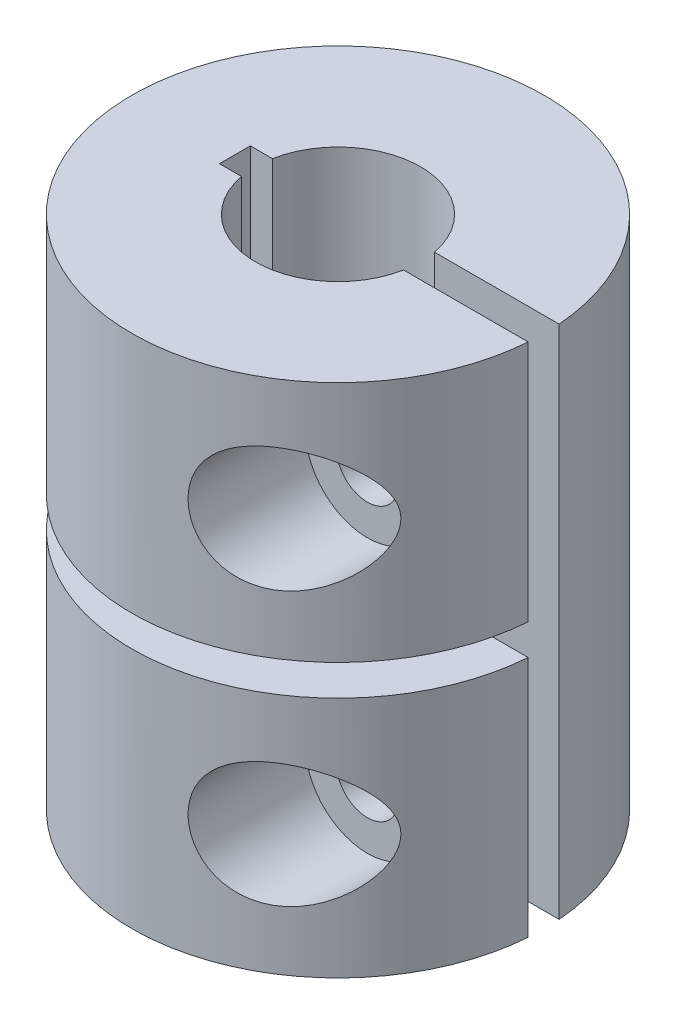
from build123d import *

# Parameters (mm, degrees)
SKETCH2_R               = 10
SKETCH2_R_2             = 4
BOSS_EXTRUDE1_DEPTH     = 25
CUT_EXTRUDE1_DEPTH      = 25
CUT_EXTRUDE1_DEPTH_BACK = 25
SKETCH3_W               = 10.75
SKETCH3_H               = 1.5
SKETCH4_W               = 17.874578158
SKETCH4_H               = 1.5
CUT_EXTRUDE2_DEPTH      = 29.722813233
SKETCH5_R               = 3
CUT_EXTRUDE3_DEPTH      = 6
SKETCH6_R               = 1.5
CUT_EXTRUDE4_DEPTH      = 4
M3_TAPPED_HOLE3_D       = 2.5


with BuildPart() as part:
    # Sketch2 → Boss-Extrude1 (new body)
    with BuildSketch(Plane(origin=(0, 0, 0), x_dir=(1, 0, 0), z_dir=(0, 1, 0))):
        with Locations(Location((0, 0, 0), (0, 0, 270))):
            Circle(SKETCH2_R)
        with Locations(Location((0, 0, 0), (0, 0, 270))):
            Circle(SKETCH2_R_2, mode=Mode.SUBTRACT)
    extrude(amount=BOSS_EXTRUDE1_DEPTH)

    # Sketch3 → Cut-Extrude1 (cut, two sides: drawn at the far end of the back side and taken through both)
    with BuildSketch(Plane(origin=(0, 0, 0), x_dir=(0, 0, -1), z_dir=(1, 0, 0)).offset(-CUT_EXTRUDE1_DEPTH_BACK)):
        with Locations((-4.625, 12.5)):
            Rectangle(SKETCH3_W, SKETCH3_H)
    extrude(amount=CUT_EXTRUDE1_DEPTH + CUT_EXTRUDE1_DEPTH_BACK, mode=Mode.SUBTRACT)

    # Sketch4 → Cut-Extrude2 (cut, through all)
    with BuildSketch(Plane(origin=(0, 25, 0), x_dir=(1, 0, 0), z_dir=(0, 1, 0))):
        with Locations((3.937289079, 0)):
            Rectangle(SKETCH4_W, SKETCH4_H)
    extrude(amount=-CUT_EXTRUDE2_DEPTH, mode=Mode.SUBTRACT)

    # Sketch5 → Cut-Extrude3 (cut)
    with BuildSketch(Plane.XY.offset(10)):
        with Locations((5.429058411, 19.125)):
            Circle(SKETCH5_R)
        with Locations((5.429058411, 5.875)):
            Circle(SKETCH5_R)
    extrude(amount=-CUT_EXTRUDE3_DEPTH, mode=Mode.SUBTRACT)

    # Sketch6 → Cut-Extrude4 (cut)
    with BuildSketch(Plane.XY.offset(4)):
        with Locations((5.429058411, 5.875)):
            Circle(SKETCH6_R)
        with Locations((5.429058411, 19.125)):
            Circle(SKETCH6_R)
    extrude(amount=-CUT_EXTRUDE4_DEPTH, mode=Mode.SUBTRACT)

    # M3 Tapped Hole3 (through all)
    with Locations(Plane.XY.offset(-0.75)):
        with Locations((5.429058411, 19.125), (5.429058411, 5.875)):
            Hole(M3_TAPPED_HOLE3_D / 2)


solid = part.part
